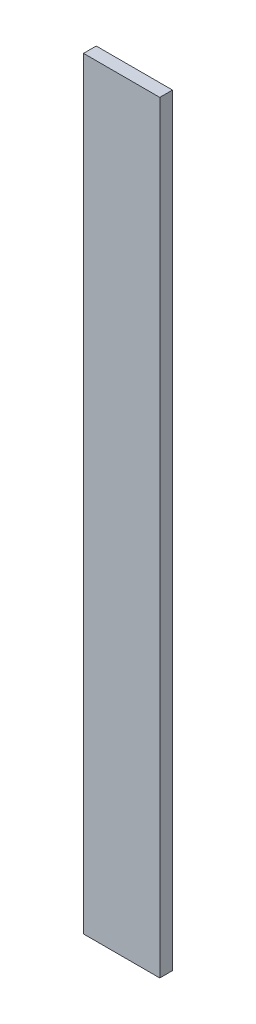
from build123d import *

# Parameters (mm, degrees)
SKETCH1_W           = 60
SKETCH1_H           = 600
BOSS_EXTRUDE1_DEPTH = 10


with BuildPart() as part:
    # Sketch1 → Boss-Extrude1 (new body)
    with BuildSketch(Plane.XY):
        with Locations((30, 300)):
            Rectangle(SKETCH1_W, SKETCH1_H)
    extrude(amount=BOSS_EXTRUDE1_DEPTH)


solid = part.part
